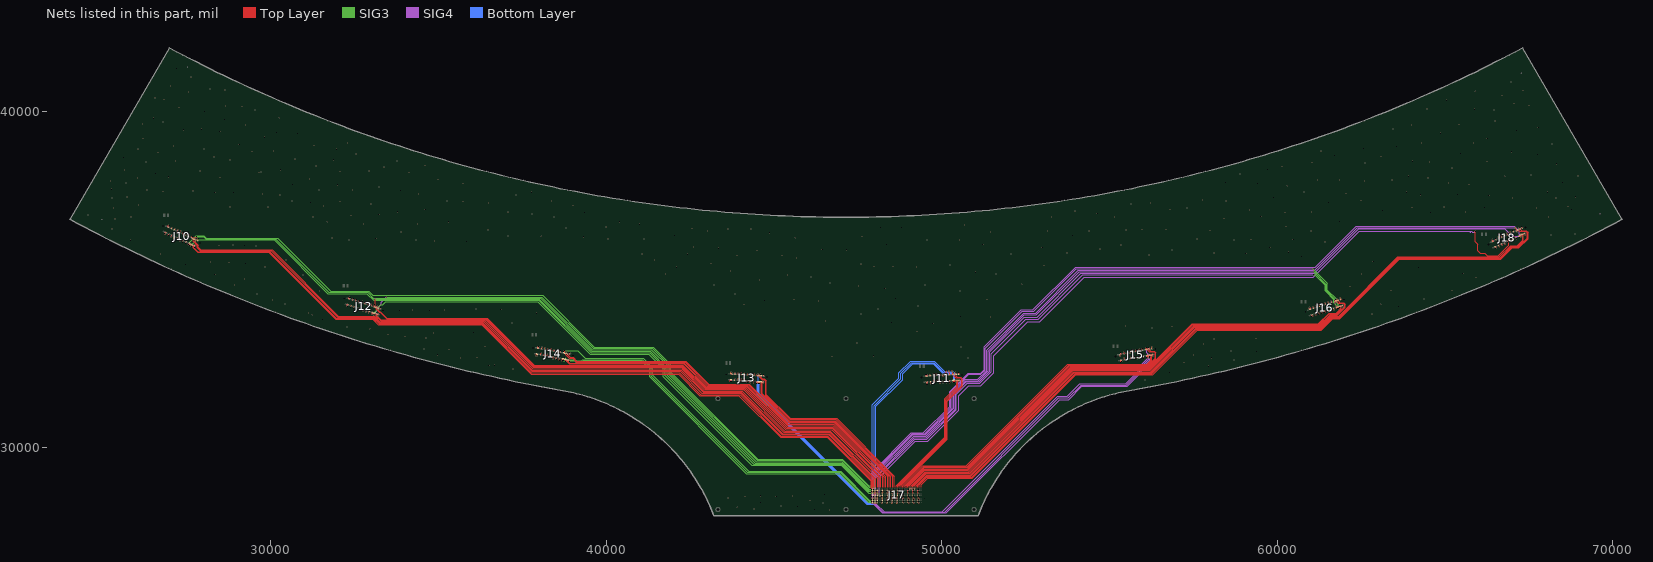
[diagram p0: the nets of this part, all layers, seen from the top]
# Altium PCB MISC86329.PcbDoc (part 10 of 11)
Units mil, origin at the board's own origin, x right, y up, seen from the top; angles counter-clockwise.
Board outline 46247.15 x 13937.21 mil, 6 copper layers (Top Layer, GND2, SIG3, SIG4, POWER5, Bottom Layer); 17 components, 210 nets, 908 pads, 1109 vias.

## Via types
v1: diameter 24, hole 12, Top Layer to Bottom Layer, 684 vias
v2: diameter 18, hole 9, Top Layer to Bottom Layer, 425 vias

## Nets (pads, with @x,y where several pads share a name; then routed paths per layer and width w, separated by ;. In a path a pad name is that pad's centre, name@x,y a point inside that pad or via, vN(x,y) a via of type N, cw(c..) or ccw(c..) an arc to the next point about the centre after c; other vN are vias at no path point) (continued)
DATAIN7P_CH7: J17.E25 J18.33 | length 23898
  Top Layer w5: v2(48164.09,28545) J17.E25@48187.89,28568.8 ; v2(65902.5,36445) 65896,36438.5 65896,36133.14 65970,36059.14 65970,35864 66043,35791 66184,35791 66255,35720 66589,35720 66898,36029 66898,36137.81 J18.33@66876.69,36159.11
  SIG4 w5: v2(48164.09,28545) 48144.09,28565 48144.09,29115.09 49215,30186 49587.14,30186 50507,31105.86 50507,31548 50807,31848 51168.14,31848 51552,32231.86 51552,32735 52571,33754 52922.14,33754 54244.14,35076 61077.14,35076 62441.14,36440 65673,36440 65741,36440 65746,36435 65746,36416.14 65751,36411.14 65761,36411.14 65766,36416.14 65766,36435 65771,36440 65776,36440 65786.86,36440 65815.86,36411 65882,36411 65896,36425 65896,36438.5
DGND: J10.5 J10.6 J10.7 J10.8 J10.13 J10.14 J10.19 J10.20 J10.25 J10.26 J10.31 J10.32 J10.37 J10.38 J10.43 J10.44 J10.49 J10.50 J10.55 J10.56 J10.61 J10.62 J10.67 J10.68 J11.5 J11.6 J11.7 J11.8 J11.13 J11.14 J11.19 J11.20 J11.25 J11.26 J11.31 J11.32 J11.37 J11.38 J11.43 J11.44 J11.49 J11.50 J11.55 J11.56 J11.61 J11.62 J11.67 J11.68 J12.5 J12.6 J12.7 J12.8 J12.13 J12.14 J12.19 J12.20 J12.25 J12.26 J12.31 J12.32 J12.37 J12.38 J12.43 J12.44 J12.49 J12.50 J12.55 J12.56 J12.61 J12.62 J12.67 J12.68 J13.5 J13.6 J13.7 J13.8 J13.13 J13.14 J13.19 J13.20 J13.25 J13.26 J13.31 J13.32 J13.37 J13.38 J13.43 J13.44 J13.49 J13.50 J13.55 J13.56 J13.61 J13.62 J13.67 J13.68 J14.5 J14.6 J14.7 J14.8 J14.13 J14.14 J14.19 J14.20 J14.25 J14.26 J14.31 J14.32 J14.37 J14.38 J14.43 J14.44 J14.49 J14.50 J14.55 J14.56 J14.61 J14.62 J14.67 J14.68 J15.5 J15.6 J15.7 J15.8 J15.13 J15.14 J15.19 J15.20 J15.25 J15.26 J15.31 J15.32 J15.37 J15.38 J15.43 J15.44 J15.49 J15.50 J15.55 J15.56 J15.61 J15.62 J15.67 J15.68 J16.5 J16.6 J16.7 J16.8 J16.13 J16.14 J16.19 J16.20 J16.25 J16.26 J16.31 J16.32 J16.37 J16.38 J16.43 J16.44 J16.49 J16.50 J16.55 J16.56 J16.61 J16.62 J16.67 J16.68 J17.A3 J17.A6 J17.A9 J17.A12 J17.A15 J17.A18 J17.A21 J17.A24 J17.A27 J17.B3 J17.B6 J17.B9 J17.B12 J17.B15 J17.B18 J17.B21 J17.B24 J17.B27 J17.C3 J17.C6 J17.C9 J17.C12 J17.C15 J17.C18 J17.C21 J17.C24 J17.C27 J17.D3 J17.D6 J17.D9 J17.D12 J17.D15 J17.D18 J17.D21 J17.D24 J17.D27 J17.E3 J17.E6 J17.E9 J17.E12 J17.E15 J17.E18 J17.E21 J17.E24 J17.E27 J17.F3 J17.F6 J17.F9 J17.F12 J17.F15 J17.F18 J17.F21 J17.F24 J17.F27 J17.G3 J17.G6 J17.G9 J17.G12 J17.G15 J17.G18 J17.G21 J17.G24 J17.G27 J17.H3 J17.H6 J17.H9 J17.H12 J17.H15 J17.H18 J17.H21 J17.H24 J17.H27 J17.J5 J17.J6 J17.J7 J17.J8 J18.5 J18.6 J18.7 J18.8 J18.13 J18.14 J18.19 J18.20 J18.25 J18.26 J18.31 J18.32 J18.37 J18.38 J18.43 J18.44 J18.49 J18.50 J18.55 J18.56 J18.61 J18.62 J18.67 J18.68 | length 12583.5
  Top Layer w5: J17.J8@49037.89,28768.8 v2(49061.69,28792.61) ; J17.F3@49287.89,28618.8 v2(49311.69,28642.61) ; J17.G3@49287.89,28668.8 v2(49311.69,28692.61) ; J17.H3@49287.89,28718.8 v2(49311.69,28742.61)
  Top Layer w20: v1(26840,36370) 26844,36376 J10.5@26861.63,36414.76 ; v1(26870,36360) 26873,36364 J10.7@26890.27,36401.67 ; J10.6@26935.3,36575.89 26952,36612 v1(26958,36627) ; v1(26956,36322) 26961,36330 J10.13@26976.21,36362.38 ; J10.8@26963.94,36562.79 26990,36616 v1(26990,36615) ; v1(27042,36280) 27049,36295 J10.19@27062.14,36323.09 ; J10.14@27049.87,36523.5 27066,36557 v1(27069,36563) ; v1(27126,36242) 27135,36257 J10.25@27148.07,36283.8 ; J10.20@27135.81,36484.21 27152,36519 v1(27156,36527) ; v1(27214,36201) 27219,36212 J10.31@27234,36244.51 ; J10.26@27221.74,36444.92 27238,36480 v1(27243,36490) ; v1(27298,36158) 27306,36175 J10.37@27319.94,36205.22 ; J10.32@27307.67,36405.64 27326,36445 v1(27331,36454) ; v1(27384,36119) 27390,36132 J10.43@27405.87,36165.94 ; J10.38@27393.6,36366.35 27414,36409 v1(27415,36411) ; v1(27471,36080) 27476,36091 J10.49@27491.8,36126.65 ; J10.44@27479.54,36327.06 27498,36368 v1(27502,36377) ; v1(27557,36042) 27563,36054 J10.55@27577.74,36087.36 ; J10.50@27565.47,36287.77 v1(27586,36332) ; J10.56@27651.4,36248.48 27671,36291 v1(27673,36295) ; v1(27654,35988) 27654,36027 J10.61@27663.67,36048.07 ; J10.62@27737.33,36209.19 27755,36247 v1(27756,36246) ; v1(27742,35960) 27742,35992 J10.67@27749.6,36008.78 ; J10.68@27823.27,36169.9 27846,36223 v1(27848,36226) ; v1(32268,34222) 32272,34232 J12.5@32282.85,34264.68 ; v1(32297,34208) 32302,34222 J12.7@32312.88,34255.17 ; J12.6@32336.33,34433.58 32351,34478 v1(32352,34479) ; J12.8@32366.36,34424.07 32380,34464 v1(32382,34471) ; v1(32388,34181) 32393,34194 J12.13@32402.96,34226.65 ; J12.14@32456.44,34395.55 32466,34426 v1(32471,34441) ; v1(32477,34150) 32481,34162 J12.19@32493.04,34198.13 ; J12.20@32546.52,34367.03 32559,34406 v1(32562,34414) ; v1(32567,34125) 32570,34131 J12.25@32583.12,34169.6 ; J12.26@32636.6,34338.5 32649,34375 v1(32653,34385) ; v1(32660,34098) 32664,34112 J12.31@32673.2,34141.08 ; J12.32@32726.68,34309.98 32740,34352 v1(32743,34361) ; v1(32750,34071) 32754,34083 J12.37@32763.28,34112.56 ; J12.38@32816.76,34281.46 32826,34311 v1(32834,34334) ; v1(32838,34034) 32842,34048 J12.43@32853.36,34084.03 ; J12.44@32906.84,34252.94 32919,34290 v1(32926,34310) ; v1(32927,34004) 32933,34022 J12.49@32943.44,34055.51 ; J12.50@32996.92,34224.41 33010,34264 v1(33016,34283) ; v1(33016,33978) 33020,33987 J12.55@33033.52,34026.99 ; J12.56@33087,34195.89 33097,34229 v1(33097,34256) ; v1(33111,33959) 33111,33961 J12.61@33123.6,33998.47 ; J12.62@33177.08,34167.37 33189,34204 v1(33193,34215) ; v1(33200,33927) 33203,33935 J12.67@33213.68,33969.94 ; J12.68@33267.16,34138.84 33279,34174 v1(33281,34176) ; v1(37915,32737) 37921,32763 J14.5@37925.69,32791.31 ; v1(37945,32733) 37949,32748 J14.7@37956.65,32785.53 ; J14.6@37958.19,32965.47 37965,33005 v1(37967,33014) ; J14.8@37989.15,32959.69 37994,32987 v1(37998,33008) ; J14.13@38049.54,32768.2 38049.54,32788.54 v1(38079,32818) ; J14.14@38082.04,32942.36 v1(38091,32993) ; J14.19@38142.42,32750.86 38142.42,32769.42 v1(38172,32799) ; J14.20@38174.92,32925.02 v1(38174.92,32978.92) ; J14.25@38235.31,32733.53 38235.31,32758.31 v1(38260,32783) ; J14.26@38267.81,32907.69 v1(38267.81,32957.19) ; J14.31@38328.19,32716.2 38328.19,32745.19 v1(38353,32770) ; J14.32@38360.69,32890.36 v1(38360.69,32938.31) ; v1(38421.08,32646.92) J14.37@38421.08,32698.87 ; J14.38@38453.58,32873.03 v1(38453.58,32921.58) ; v1(38513.96,32626.04) J14.43@38513.96,32681.53 ; J14.44@38546.46,32855.69 v1(38546.46,32904.54) ; v1(38606.85,32603.15) J14.49@38606.85,32664.2 ; J14.50@38639.35,32838.36 v1(38639.35,32889.35) ; v1(38685,32591) 38699.73,32605.73 J14.55@38699.73,32646.87 ; J14.56@38732.23,32821.03 v1(38732.23,32870.23) ; v1(38792.62,32562.38) J14.61@38792.62,32629.54 ; J14.62@38825.12,32803.7 v1(38825.12,32851.88) ; J14.67@38885.5,32612.2 38885.5,32582.5 v1(38911,32557) ; J14.68@38918,32786.36 v1(38918,32833) ; v1(43703,31968) J13.5@43706.03,32016.6 ; J13.6@43717.06,32193.43 43720,32239 v1(43721,32250) ; v1(43735,31963) 43735,31971 J13.7@43737.46,32014.64 ; J13.8@43748.5,32191.46 43751,32234 v1(43751,32239) ; J13.13@43831.77,32008.76 v1(43834,32052) ; J13.14@43842.8,32185.58 43846,32231 v1(43846,32232) ; J13.19@43926.07,32002.88 43929,32049 v1(43929,32050) ; J13.20@43937.11,32179.7 43940,32223 v1(43940,32227) ; J13.25@44020.38,31996.99 44023,32042 v1(44024,32047) ; J13.26@44031.41,32173.81 44034,32217 v1(44035,32224) ; J13.31@44114.68,31991.11 v1(44118,32044) ; J13.32@44125.72,32167.93 44130,32214 v1(44130,32217) ; v1(44206,31936) 44207,31947 J13.37@44208.99,31985.22 ; J13.38@44220.02,32162.05 44223,32207 v1(44224,32209) ; v1(44300,31928) 44300,31933 J13.43@44303.29,31979.34 ; J13.44@44314.33,32156.16 44317,32198 v1(44318,32203) ; v1(44394,31922) 44395,31935 J13.49@44397.6,31973.46 ; J13.50@44408.63,32150.28 44412,32196 v1(44413,32200) ; v1(44488,31915) J13.55@44491.9,31967.57 ; J13.56@44502.94,32144.4 v1(44505,32184) ; v1(44583,31914) 44584,31924 J13.61@44586.21,31961.69 ; J13.62@44597.24,32138.51 v1(44600,32186) ; v1(44678,31908) 44679,31918 J13.67@44680.51,31955.81 ; J13.68@44691.54,32132.63 44694,32173 v1(44695,32181) ; v2(48064.09,28345) J17.A27@48087.89,28368.8 ; v2(48064.09,28395) J17.B27@48087.89,28418.8 ; v2(48064.09,28445) J17.C27@48087.89,28468.8 ; v2(48064.09,28495) J17.D27@48087.89,28518.8 ; v2(48064.09,28545) J17.E27@48087.89,28568.8 ; v2(48064.09,28642.61) J17.F27@48087.89,28618.8 ; v2(48064.09,28692.61) J17.G27@48087.89,28668.8 ; v2(48064.09,28742.61) J17.H27@48087.89,28718.8 ; v2(48214.09,28345) J17.A24@48237.89,28368.8 ; v2(48214.09,28395) J17.B24@48237.89,28418.8 ; v2(48214.09,28445) J17.C24@48237.89,28468.8 ; v2(48214.09,28495) J17.D24@48237.89,28518.8 ; v2(48214.09,28545) J17.E24@48237.89,28568.8 ; v2(48214.09,28642.61) J17.F24@48237.89,28618.8 ; v2(48214.09,28692.61) J17.G24@48237.89,28668.8 ; v2(48214.09,28742.61) J17.H24@48237.89,28718.8 ; v2(48364.09,28345) J17.A21@48387.89,28368.8 ; v2(48364.09,28395) J17.B21@48387.89,28418.8 ; v2(48364.09,28445) J17.C21@48387.89,28468.8 ; v2(48364.09,28495) J17.D21@48387.89,28518.8 ; v2(48364.09,28545) J17.E21@48387.89,28568.8 ; v2(48364.09,28642.61) J17.F21@48387.89,28618.8 ; v2(48364.09,28692.61) J17.G21@48387.89,28668.8 ; v2(48364.09,28742.61) J17.H21@48387.89,28718.8 ; v2(48514.09,28345) J17.A18@48537.89,28368.8 ; v2(48514.09,28395) J17.B18@48537.89,28418.8 ; v2(48514.09,28445) J17.C18@48537.89,28468.8 ; v2(48514.09,28495) J17.D18@48537.89,28518.8 ; v2(48514.09,28545) J17.E18@48537.89,28568.8 ; v2(48514.09,28642.61) J17.F18@48537.89,28618.8 ; v2(48514.09,28692.61) J17.G18@48537.89,28668.8 ; v2(48514.09,28742.61) J17.H18@48537.89,28718.8 ; v2(48664.09,28345) J17.A15@48687.89,28368.8 ; v2(48664.09,28395) J17.B15@48687.89,28418.8 ; v2(48664.09,28445) J17.C15@48687.89,28468.8 ; v2(48664.09,28495) J17.D15@48687.89,28518.8 ; v2(48664.09,28545) J17.E15@48687.89,28568.8 ; J17.F15@48687.89,28618.8 v2(48711.69,28642.61) ; J17.G15@48687.89,28668.8 v2(48711.69,28692.61) ; J17.H15@48687.89,28718.8 v2(48711.69,28742.61) ; J17.A12@48837.89,28368.8 v2(48861.69,28345) ; J17.B12@48837.89,28418.8 v2(48861.69,28395) ; J17.C12@48837.89,28468.8 v2(48861.69,28445) ; J17.D12@48837.89,28518.8 v2(48861.69,28495) ; J17.E12@48837.89,28568.8 v2(48861.69,28545) ; J17.F12@48837.89,28618.8 v2(48861.69,28642.61) ; J17.G12@48837.89,28668.8 v2(48861.69,28692.61) ; J17.H12@48837.89,28718.8 v2(48861.69,28742.61) ; J17.A9@48987.89,28368.8 v2(49011.69,28345) ; J17.B9@48987.89,28418.8 v2(49011.69,28395) ; J17.C9@48987.89,28468.8 v2(49011.69,28445) ; J17.D9@48987.89,28518.8 v2(49011.69,28495) ; J17.E9@48987.89,28568.8 v2(49011.69,28545) ; J17.F9@48987.89,28618.8 v2(49011.69,28642.61) ; J17.G9@48987.89,28668.8 v2(49011.69,28692.61) ; J17.H9@48987.89,28718.8 v2(49011.69,28742.61) ; J17.J8@49037.89,28768.8 v2(49061.69,28792.61) ; J17.J7@49087.89,28768.8 v2(49111.69,28792.61) ; J17.A6@49137.89,28368.8 v2(49161.69,28345) ; J17.B6@49137.89,28418.8 v2(49161.69,28395) ; J17.C6@49137.89,28468.8 v2(49161.69,28445) ; J17.D6@49137.89,28518.8 v2(49161.69,28495) ; J17.E6@49137.89,28568.8 v2(49161.69,28545) ; J17.F6@49137.89,28618.8 v2(49161.69,28642.61) ; J17.G6@49137.89,28668.8 v2(49161.69,28692.61) ; J17.H6@49137.89,28718.8 v2(49161.69,28742.61) ; J17.J6@49137.89,28768.8 v2(49161.69,28792.61) ; J17.J5@49187.89,28768.8 v2(49211.69,28792.61) ; J17.A3@49287.89,28368.8 v2(49311.69,28345) ; J17.B3@49287.89,28418.8 v2(49311.69,28395) ; J17.C3@49287.89,28468.8 v2(49311.69,28445) ; J17.D3@49287.89,28518.8 v2(49311.69,28495) ; J17.E3@49287.89,28568.8 v2(49311.69,28545) ; J17.F3@49287.89,28618.8 v2(49311.69,28642.61) ; J17.G3@49287.89,28668.8 v2(49311.69,28692.61) ; J17.H3@49287.89,28718.8 v2(49311.69,28742.61) ; v1(49526,32172) 49525,32168 J11.6@49527.1,32128.97 ; J11.5@49537.7,31952.12 49541,31892 v1(49542,31888) ; v1(49555,32178) 49556,32171 J11.8@49558.54,32130.85 ; J11.7@49569.14,31954.01 49573,31892 v1(49574,31886) ; v1(49651,32183) 49651,32177 J11.14@49652.86,32136.51 ; J11.13@49663.45,31959.66 49667,31901 v1(49667,31896) ; v1(49744,32187) J11.20@49747.17,32142.16 ; v1(49754,32026) J11.19@49757.77,31965.31 ; v1(49839,32198) 49839,32197 J11.26@49841.49,32147.81 ; v1(49849,32028) 49849,32025 J11.25@49852.09,31970.97 ; v1(49933,32202) J11.32@49935.81,32153.47 ; J11.31@49946.41,31976.62 49949,31924 v1(49949,31923) ; J11.38@50030.13,32159.12 50032,32118 v1(50034,32112) ; J11.37@50040.73,31982.27 50044,31930 v1(50045,31926) ; v1(50118,32290) 50118,32288 J11.44@50124.45,32164.77 ; J11.43@50135.05,31987.92 50138,31938 v1(50139,31930) ; v1(50213,32285) 50213,32279 J11.50@50218.77,32170.43 ; J11.49@50229.37,31993.58 50232,31946 v1(50233,31936) ; v1(50307,32287) 50307,32282 J11.56@50313.09,32176.08 ; J11.55@50323.69,31999.23 50327,31961 v1(50328,31956) ; v1(50404,32244) 50404,32240 J11.62@50407.41,32181.73 ; J11.61@50418.01,32004.88 50420,31963 v1(50421,31956) ; v1(50499,32234) J11.68@50501.73,32187.38 ; J11.67@50512.33,32010.54 50515,31970 v1(50515,31968) ; J15.6@55301.68,32773.06 55309,32733 v1(55310,32727) ; v1(55323,32828) 55325,32821 J15.8@55332.65,32778.76 ; v1(55333.75,32539.75) J15.5@55333.75,32598.82 ; v1(55364.73,32561.73) J15.7@55364.73,32604.52 ; v1(55418,32842) 55421,32823 J15.14@55425.58,32795.87 ; v1(55426,32670) 55457.65,32638.35 J15.13@55457.65,32621.63 ; J15.20@55518.51,32812.97 55518.51,32766.49 55518.99,32766.01 v1(55519,32765) ; v1(55526,32683) 55550.58,32658.42 J15.19@55550.58,32638.73 ; J15.26@55611.44,32830.08 v1(55611.44,32876.44) ; v1(55621,32702) 55643.51,32679.49 J15.25@55643.51,32655.84 ; J15.32@55704.36,32847.18 v1(55704.36,32900.36) ; J15.31@55736.44,32672.95 v1(55736.44,32719.44) ; J15.38@55797.29,32864.29 v1(55797.29,32917.29) ; v1(55829.36,32643.36) J15.37@55829.36,32690.05 ; J15.44@55890.22,32881.39 v1(55890.22,32932.22) ; v1(55922.29,32648.29) J15.43@55922.29,32707.16 ; J15.50@55983.14,32898.5 v1(55983.14,32945.14) ; v1(56015.22,32662.22) J15.49@56015.22,32724.26 ; J15.56@56076.07,32915.61 v1(56076.07,32962.07) ; v1(56108.14,32689.14) J15.55@56108.14,32741.37 ; J15.62@56169,32932.71 v1(56169,32978) ; v1(56201.07,32711.07) J15.61@56201.07,32758.47 ; J15.68@56261.92,32949.82 v1(56261.92,32997.92) ; v1(56294,32726) J15.67@56294,32775.58 ; v1(60943,34154) 60945,34147 J16.6@60954.72,34116.09 ; v1(60964,34185) 60965.24,34182.1 60970,34171 ; v1@60965,34182 60976.06,34152.34 J16.8@60984.77,34125.53 ; J16.5@61007.79,33947.06 61020,33910 v1(61023,33902) ; J16.7@61037.84,33956.5 61050,33920 v1(61052,33915) ; v1(61060,34199) 61064,34187 J16.14@61074.92,34153.83 ; J16.13@61127.99,33984.8 61139,33951 v1(61141,33947) ; v1(61150,34230) 61154,34218 J16.20@61165.07,34182.13 ; J16.19@61218.14,34013.1 61228,33981 v1(61231,33972) ; v1(61238,34261) 61242,34253 J16.26@61255.22,34210.44 ; J16.25@61308.29,34041.4 61320,34005 v1(61321,34000) ; v1(61331,34281) 61331,34282 J16.32@61345.37,34238.74 ; J16.31@61398.44,34069.71 61409,34038 v1(61415,34021) ; v1(61418,34320) 61421,34312 J16.38@61435.52,34267.04 ; J16.37@61488.59,34098.01 61499,34067 v1(61507,34046) ; v1(61508,34345) 61515,34329 J16.44@61525.67,34295.34 ; J16.43@61578.74,34126.31 61591,34089 v1(61596,34075) ; v1(61602,34366) 61606,34355 J16.50@61615.82,34323.65 ; J16.49@61668.89,34154.62 61678,34124 61682,34110 v1(61684,34104) ; J16.56@61705.97,34351.95 61717,34320 v1(61721,34309) ; v1(61745,34224) 61748,34216 J16.55@61759.04,34182.92 ; v1(61782,34423) J16.62@61796.12,34380.25 ; J16.61@61849.19,34211.22 61860,34181 v1(61861,34177) ; v1(61871,34457) J16.68@61886.27,34408.56 ; J16.67@61939.34,34239.53 61952,34200 v1(61954,34195) ; v1(66383,36181) 66387,36171 J18.6@66401.96,36138.05 ; v1(66405,36207) 66410,36197 J18.8@66430.63,36151.07 ; J18.5@66475.23,35976.74 66491,35943 v1(66497,35930) ; v1(66498,36229) 66500,36224 J18.14@66516.66,36190.15 ; J18.7@66503.91,35989.77 66522,35951 v1(66524,35947) ; v1(66583,36273) 66585,36266 J18.20@66602.69,36229.23 ; J18.13@66589.93,36028.85 66604,35999 v1(66610,35987) ; v1(66670,36307) 66674,36299 J18.26@66688.72,36268.31 ; J18.19@66675.96,36067.93 v1(66697,36024) ; v1(66756,36347) 66758,36343 J18.32@66774.75,36307.39 ; J18.25@66761.99,36107.01 66780,36068 v1(66781,36064) ; v1(66840,36390) 66843,36385 J18.38@66860.78,36346.47 ; J18.31@66848.02,36146.08 66866,36109 v1(66868,36105) ; v1(66927,36429) 66930,36422 J18.44@66946.8,36385.54 ; J18.37@66934.05,36185.16 66954,36143 v1(66955,36142) ; v1(67014,36467) 67016,36462 J18.50@67032.83,36424.62 ; J18.43@67020.08,36224.24 v1(67039,36185) ; J18.49@67106.1,36263.32 67122,36230 v1(67127,36222) ; J18.56@67118.86,36463.7 67134,36433 v1(67137,36427) ; v1(67184,36546) 67187,36540 J18.62@67204.89,36502.78 ; J18.55@67192.13,36302.4 67209,36267 v1(67214,36258) ; v1(67260,36381) 67263,36374 J18.61@67278.16,36341.48 ; v1(67271,36584) 67276,36574 J18.68@67290.92,36541.86 ; J18.67@67364.19,36380.56 67383,36343 v1(67387,36333)
  other v1: 46658,28143 46206,28159 44415,28164 43908,28221 45709,28247 45207,28258 46459,28346 44607,28366 46076,28428 43639,28496 44136,28547 45072,28547 45559,28553 44601,28563 46506,28604 56058,32008 56783,32233 37223,32334 57950,32423 36505,32446 36677,32452 57216,32530 58715,32605 35667,32666 50786,32672 58039,32675 36154,32684 46731,32718 47974,32737 57499,32759 34972,32767 59378,32861 58622,32874 35322,32922 34579,32940 50579,32999 36398,33017 57804,33087 47470,33111 58123,33233 59360,33250 34627,33260 34003,33314 33504,33367 34853,33415 36047,33427 49262,33464 32957,33540 56270,33560 32286,33593 56863,33613 55479,33626 49733,33699 37200,33706 48507,33728 46544,33775 31549,33813 51453,33887 50555,33906 31246,33957 62826,33972 47591,33980 37930,34003 31129,34011 33849,34086 34734,34086 34229,34104 35191,34104 36861,34110 36124,34128 48099,34132 63611,34205 49296,34221 44104,34261 63082,34269 30433,34282 46329,34373 44721,34382 30061,34399 45604,34411 51354,34411 64372,34429 48620,34438 29599,34579 43843,34579 50544,34661 31464,34664 63387,34677 65205,34685 48304,34745 62169,34805 47526,34812 43211,34840 49508,34840 28923,34845 52387,34867 46674,34902 44572,34999 29221,35026 65918,35062 46105,35083 45400,35140 30965,35143 28339,35159 41767,35166 51619,35166 62505,35166 65525,35182 51003,35224 43709,35256 64204,35366 42094,35373 49246,35383 29832,35387 47984,35401 48554,35401 53052,35420 50252,35435 27474,35450 47595,35461 43122,35486 29258,35488 28764,35515 28211,35526 62858,35542 41440,35586 30465,35595 45672,35652 60717,35697 43899,35719 45245,35728 56184,35739 42421,35760 52068,35763 26725,35771 41079,35773 59061,35782 58121,35796 53736,35806 60339,35819 44493,35870 56868,35883 47164,35894 46441,35897 54720,35909 43348,35938 59776,35957 52998,35961 42601,35980 29572,36004 28461,36025 29232,36025 28886,36036 55335,36037 51225,36055 48358,36056 61418,36132 35837,36137 34885,36155 25831,36176 49557,36180 58710,36182 50527,36187 32344,36190 34338,36190 60476,36196 59216,36203 41126,36214 57615,36217 40058,36221 33138,36226 31841,36243 45637,36252 39324,36281 47622,36286 38069,36296 37081,36305 42034,36321 53901,36324 68159,36339 68872,36367 44871,36402 51453,36423 33896,36428 43020,36448 61011,36448 53151,36456 54398,36456 57992,36467 55500,36479 36481,36490 56680,36500 55968,36503 44310,36514 43627,36517 25274,36520 42564,36524 38810,36541 48177,36563 48805,36563 40005,36574 60257,36592 50674,36632 40993,36654 32777,36656 34382,36667 31691,36728 35308,36728 40399,36728 61853,36736 25365,36818 58415,36827 68077,36866 38450,36868 53274,36873 55147,36875 25849,36877 31267,36878 59506,36891 32405,36914 24563,36932 33226,36940 37796,36958 54634,36976 64561,37007 39357,37008 60225,37009 37081,37011 61025,37016 65611,37016 33782,37028 53967,37041 63130,37066 59166,37073 68763,37093 56801,37096 34611,37099 57307,37136 25319,37139 67718,37142 66176,37150 64014,37157 29926,37162 64975,37167 28792,37176 68660,37183 31575,37196 39017,37208 26065,37225 32988,37258 55641,37261 56217,37283 36499,37284 31197,37302 61522,37306 32070,37337 35731,37337 38376,37342 30643,37343 35265,37347 58478,37349 62499,37367 57770,37374 67012,37434 25281,37437 68297,37438 59884,37457 25732,37467 68880,37475 66300,37510 30278,37521 37311,37522 64263,37533 65373,37545 29758,37551 34408,37558 62046,37569 28903,37597 28340,37601 63855,37607 68048,37608 37782,37609 60801,37620 26802,37635 27688,37651 33879,37664 31444,37672 32449,37672 26313,37674 25266,37696 33235,37761 60296,37802 32001,37830 30657,37837 65707,37841 35740,37867 59414,37874 25694,37880 65104,37889 58460,37895 68497,37897 62604,37938 25235,37941 61197,37972 61853,37978 63425,37978 34990,37990 31161,38008 26038,38033 64490,38039 28498,38048 26962,38071 63908,38084 66778,38084 68959,38099 67564,38116 58892,38153 26580,38162 34126,38193 29656,38199 29720,38208 32070,38228 27909,38239 32944,38246 25656,38269 30301,38277 59712,38290 65205,38322 33385,38352 60141,38371 31364,38387 34603,38407 68316,38458 62609,38474 61036,38490 64539,38506 26290,38514 66249,38522 64028,38532 33773,38537 27176,38544 28796,38575 31878,38577 30736,38590 25625,38644 28319,38665 63095,38672 61699,38700 67751,38733 32555,38749 65454,38766 26649,38789 66979,38814 29453,38820 61300,38830 30086,38839 26053,38888 31964,38890 28016,38896 62566,38913 63551,38974 27115,38980 31294,38996 29071,39033 68189,39050 65841,39072 64301,39074 32299,39075 66257,39204 26206,39209 29819,39247 30805,39354 64863,39367 30184,39389 28490,39415 67126,39447 27405,39469 27948,39484 63449,39496 67775,39537 29262,39606 64000,39612 65415,39625 26183,39637 26802,39706 66494,39734 28632,39772 26519,39813 30263,39828 28039,40011 29537,40057 66453,40063 65876,40081 64463,40097 27275,40134 29155,40157 28658,40172 67499,40194 67050,40255 65040,40348 26832,40370 26557,40424 66695,40494 27558,40600 65900,40616 67324,40643 28639,40655 28200,40684 27016,40775 66963,40892 27627,41035 27199,41295
  other v2: 49311.69,28642.61 49311.69,28692.61 49311.69,28742.61 49061.69,28792.61
IO0_CH0: J10.57 J17.G28 | length 24027.9
  Top Layer w5: v2(27593,36021) 27593,36050 27606.38,36063.38 J10.57@27606.38,36074.26 ; v2(48014.09,28692.61) J17.G28@48037.89,28668.8
  SIG3 w5: v2@27593,36023 27593,36110.58 27788.42,36306 28018,36306 28091,36233 28163,36233 ; 28159,36233 28163,36233 ; v2(48014.09,28692.61) 47997.59,28709.11 47997.59,28793.41 47972,28819 47954,28819 47940,28833 47940,28851 47924,28867 47829,28867 47040,29656 44524,29656 41934,32246 41934,32465 41404,32995 39651,32995 38111,34535 33044,34535 32928,34651 31798,34651 30216,36233 28163,36233
IO0_CH1: J12.57 J17.F28 | length 17930.8
  Top Layer w5: v2(33055,33969) 33055,34008.93 J12.57@33063.55,34017.48 ; v2(48014.09,28642.61) J17.F28@48037.89,28618.8
  SIG4 w5: v2@33059,33972 33225,34138 33225,34187 33303,34265 33303,34332 v2(33457,34486)
  SIG3 w5: v2(33457,34486) 38088,34486 39615,32959 41379,32959 41894,32444 41894,32221 44498,29617 47032,29617 47836,28813 47925,28813 47939,28799 47939,28785 47955,28769 47973,28769 47986,28756 47986,28670.69 v2(48014.09,28642.61)
IO0_CH2: J14.57 J17.B28 | length 11301.6
  Top Layer w5: v2@38725,32593 38725,32634 38730.69,32639.69 J14.57@38730.69,32641.09 ; v2(48014.09,28395) J17.B28@48037.89,28418.8
  SIG4 w5: v2@38723,32591 v2(38724,32590)
  SIG3 w5: v2(38724,32590) 39053,32590 39080,32563 39290,32563 39317,32590 41054,32590 41298,32346 41298,32105 44176,29227 46957,29227 47819,28365 47984.09,28365 v2(48014.09,28395)
IO0_CH3: J13.57 J17.A28 | length 5297.8
  Top Layer w5: v2@44523.34,31910.34 J13.57@44523.34,31965.61 ; v2(48014.09,28345) J17.A28@48037.89,28368.8
  Bottom Layer w5: v2@44520,31906 44510,31896 44510,31572 47772,28310 47979.09,28310 v2(48014.09,28345) ; v2@44521,31906 v2(44521,31907)
IO0_CH4: J11.57 J17.H28 | length 5891.1
  Top Layer w5: v2(48014.09,28742.61) J17.H28@48037.89,28718.8 ; v2(50355.13,31939.13) J11.57@50355.13,32001.12
  Bottom Layer w5: v2(48014.09,28742.61) 48038,28766.52 48038,31230 48836,32028 48836,32193 49139,32496 49746,32496 50046,32196 50319,32196 50355.13,32159.87 v2(50355.13,31939.13)
IO0_CH5: J15.57 J17.C28 | length 10400.7
  Top Layer w5: v2(48014.09,28445) J17.C28@48037.89,28468.8 ; v2(56139.12,32666.12) J15.57@56139.12,32747.07
  SIG4 w5: v2(48014.09,28445) 48042,28417.09 48042,28331 48286,28087 50021,28087 53461,31527 53747,31527 54116,31896 55482,31896 55857,32271 55857,32385 v2@56138,32666
IO0_CH6: J16.57 J17.D28 | length 18151.7
  Top Layer w5: v2(48014.09,28495) J17.D28@48037.89,28518.8 ; v2(61789.09,34137.91) J16.57@61789.09,34192.35
  SIG4 w5: v2(48014.09,28495) 48042,28522.91 48042,29094 49199,30251 49560,30251 50441,31132 50441,31591 50769,31919 51141,31919 51482,32260 51482,32795 52509,33822 52884,33822 54210,35148 v2(61074,35148)
  SIG3 w5: v2@61070,35148 v2(61074,35148) 61109,35148 61422,34835 61422,34671 61686.5,34406.5 61686.5,34315.92 61712.92,34289.5 61713.5,34289.5 61789,34214 ; v2(61789.09,34137.91) 61789.09,34214
IO0_CH7: J17.E28 J18.57 | length 23718.6
  Top Layer w5: v2(48014.09,28545) J17.E28@48037.89,28568.8 ; J18.57@67220.81,36315.42 67220.81,36302.19 v2@67257,36266 ; v2(67258,36266) v2@67257,36266 ; v2@67259,36264 v2@67257,36266
  SIG4 w5: v2(48014.09,28545) 48032,28562.91 48032,28888 ; 48032,28895 48032,28888 ; v2(67258,36266) 67223,36301 67003,36301 66784,36520 62430,36520 61101,35191 54143,35191 52842,33890 52464,33890 51425,32851 51425,32268 51116,31959 50739,31959 50398,31618 50398,31149 49540,30291 49178,30291 48032,29145 48032,28888
IO1_CH0: J10.58 J17.G29 | length 23611.7
  Top Layer w5: J10.58@27690,36245.34 27715.66,36271 27786,36271 v2(27799,36284) ; v2(47964.09,28692.61) J17.G29@47987.89,28668.8
  SIG3 w5: v2@27800,36283 28012,36283 28084,36211 30156,36211 31744,34623 32896,34623 33066,34453 38055,34453 39586,32922 41344,32922 41846,32420 41846,32204 44477,29573 47028,29573 47837,28764 47924,28764 47946,28742 47946,28710.69 v2(47964.09,28692.61)
IO1_CH1: J12.58 J17.F29 | length 17648.8
  Top Layer w5: J12.58@33117.03,34186.38 33117.03,34419.03 v2@33121,34423 ; v2(47964.09,28642.61) J17.F29@47987.89,28618.8
  SIG3 w5: v2@33117,34423 38016,34423 39574,32865 41316,32865 41796,32385 41796,32179 44443,29532 47022,29532 47840,28714 47918,28714 47941.85,28690.15 47941.85,28664.85 v2(47964.09,28642.61)
  other v2: 33116,34424
IO1_CH2: J14.58 J17.B29 | length 11294.3
  Top Layer w5: J14.58@38763.19,32815.25 38768,32820.06 38768,32884 v2@38766,32886 ; v2(47964.09,28395) J17.B29@47987.89,28418.8
  SIG3 w5: v2(38768,32889) 39152,32889 39386,32655 41102,32655 41387,32370 41387,32149 44244,29292 46987,29292 47860,28419 47940.09,28419 v2(47964.09,28395)
IO1_CH3: J13.58 J17.A29 | length 5474
  Top Layer w5: J13.58@44534.37,32142.43 v2(44534.37,32193.37) ; v2(47964.09,28345) J17.A29@47987.89,28368.8
  Bottom Layer w5: v2@44535,32189 44538.27,32185.73 44538.27,31585.73 47799,28325 47944.09,28325 v2(47964.09,28345)
IO1_CH4: J11.58 J17.H29 | length 5714.2
  Top Layer w5: v2(47964.09,28742.61) J17.H29@47987.89,28718.8 ; J11.58@50344.53,32177.96 v2(50344.53,32230.47)
  Bottom Layer w5: v2(47964.09,28742.61) 47988,28766.52 47988,31252 48781,32045 48781,32208 49107,32534 49765,32534 50068.53,32230.47 v2(50344.53,32230.47)
IO1_CH5: J15.58 J17.C29 | length 10818.9
  Top Layer w5: v2(47964.09,28445) J17.C29@47987.89,28468.8 ; J15.58@56107.05,32921.31 v2(56107.05,32976.05)
  SIG4 w5: v2(47964.09,28445) 47990,28419.09 47990,28330 48249,28071 50085,28071 53495,31481 53773,31481 54153,31861 55504,31861 55900,32257 55900,32370 56166,32636 56166,32772 56108,32830 56108,32975 v2@56109,32976
IO1_CH6: J16.58 J17.D29 | length 18077.8
  Top Layer w5: v2(47964.09,28495) J17.D29@47987.89,28518.8 ; v2(61730,34411) 61730,34367.41 J16.58@61736.02,34361.38
  SIG4 w5: v2(47964.09,28495) 47993,28523.91 47993,29169 49163,30339 49525,30339 50354,31168 50354,31629 50723,31998 51091,31998 51382,32289 51382,32873 52462,33953 52817,33953 54099,35235 v2(61081,35235)
  SIG3 w5: v2@61080,35235 61461,34854 61461,34680 v2(61730,34411)
IO1_CH7: J17.E29 J18.58 | length 23589.8
  Top Layer w5: v2(47964.09,28545) J17.E29@47987.89,28568.8 ; v2@67078.13,36546.13 67091.13,36533.13 J18.58@67147.54,36476.73
  SIG4 w5: v2(47964.09,28545) 47981,28561.91 47981,28888 ; 47981,28892 47981,28888 ; v2(67078,36545) 67066,36557 62389,36557 61111,35279 54069,35279 52799,34009 52446,34009 51338,32901 51338,32294 51081,32037 50704,32037 50309,31642 50309,31174 49514,30379 49138,30379 47981,29222 47981,28888
IO2_CH0: J10.59 J17.G30 | length 23701.8
  Top Layer w5: v2(27626,36006) 27626,36052.14 J10.59@27635.02,36061.17 ; v2(47914.09,28692.61) J17.G30@47937.89,28668.8
  SIG3 w5: v2@27629,36008 27809,36188 27959,36188 ; 27952,36188 27959,36188 ; 28223,36188 28228,36188 ; v2@47920,28690 47917.39,28692.61 v2(47914.09,28692.61) 47816.39,28692.61 47005,29504 44394,29504 41750,32148 41750,32363 41294,32819 39556,32819 37989,34386 33077,34386 32874,34589 31708,34589 30109,36188 28228,36188 ; 27959,36188 28228,36188
IO2_CH1: J12.59 J17.F30 | length 17670.1
  Top Layer w5: v2(33086,33942) 33086,34000.4 J12.59@33093.57,34007.97 ; v2(47914.09,28642.61) J17.F30@47937.89,28618.8
  SIG3 w5: v2@33084,33946 33084,33998 33217,34131 33217,34180 33293,34256 33342,34256 33435,34349 33532,34349 ; 33528,34349 33532,34349 ; v2(47914.09,28642.61) 47828.39,28642.61 47001,29470 44341,29470 41705,32106 41705,32351 41276,32780 39530,32780 37961,34349 33532,34349
IO2_CH2: J14.59 J17.B30 | length 11163.8
  Top Layer w5: J14.59@38761.66,32635.31 38766,32639.66 v2(38766,32677) ; v2(47914.09,28395) J17.B30@47937.89,28418.8
  SIG3 w5: v2@38769,32674 38822,32621 39056,32621 39096,32581 39266,32581 39309,32624 41075,32624 41342,32357 41342,32129 44213,29258 46975,29258 47838,28395 v2(47914.09,28395)
IO2_CH3: J13.59 J17.A30 | length 5095.5
  Top Layer w5: v2(44554.77,31905.23) J13.59@44554.77,31963.65 ; v2(47914.09,28345) J17.A30@47937.89,28368.8
  Bottom Layer w5: v2@44554,31905 44565,31894 44565,31606 47826,28345 v2(47914.09,28345)
IO2_CH4: J11.59 J17.H30 | length 6147.6
  Top Layer w5: v2(47914.09,28742.61) J17.H30@47937.89,28718.8 ; v2(50386.57,31939.57) J11.59@50386.57,32003
  Bottom Layer w5: v2(47914.09,28742.61) 47937,28765.52 47937,31280 48726,32069 48726,32226 49076,32576 49773,32576 50089,32260 50342,32260 50386.57,32215.43 v2(50386.57,31939.57)
IO2_CH5: J15.59 J17.C30 | length 10634.5
  Top Layer w5: v2(47914.09,28445) J17.C30@47937.89,28468.8 ; J15.59@56170.09,32752.77 56170.09,32734.91 56178,32727 56178,32693 v2(56196,32675)
  SIG4 w5: v2(47914.09,28445) 47939,28420.09 47939,28340 48226,28053 50134,28053 53513,31432 53782,31432 54171,31821 55525,31821 55946,32242 55946,32358 56197,32609 v2@56197,32674
IO2_CH6: J16.59 J17.D30 | length 18649.1
  Top Layer w5: v2(47914.09,28495) J17.D30@47937.89,28518.8 ; v2(61819.14,34137.14) J16.59@61819.14,34201.79
  SIG4 w5: v2(47914.09,28495) 47944,28524.91 47944,29237 49120,30413 49498,30413 50271,31186 50271,31657 50801,32187 51168,32187 51291,32310 51291,32957 52397,34063 52746,34063 54010,35327 v2(61062,35327)
  SIG3 w5: v2@61061,35324 61495,34890 61495,34692 61757,34430 61757,34325 61819.14,34262.86 v2(61819.14,34137.14)
IO2_CH7: J17.E30 J18.59 | length 24056.1
  Top Layer w5: v2(47914.09,28545) J17.E30@47937.89,28568.8 ; J18.59@67249.48,36328.45 67249.48,36312.52 v2@67283,36279
  SIG4 w5: v2(47914.09,28545) 47932,28562.91 47932,29271 49100,30439 49458,30439 50237,31218 50237,31662 50791,32216 51161,32216 51267,32322 51267,33005 52365,34103 52713,34103 53988,35378 61137,35378 62349,36590 67066,36590 67214,36442 67214,36349 v2(67283,36280)
IO3_CH0: J10.60 J17.J29 | length 23613.6
  Top Layer w5: J10.60@27708.69,36222.29 27702,36215.6 27702,36141 27822,36021 27822,35955 27911,35866 28065,35866 ; 28069,35866 28065,35866 ; J17.J29@47989,28768 47965,28792 47965,29041 46630,30376 45254,30376 44014,31616 42857,31616 42205,32268 37785,32268 36330,33723 33246,33723 33081,33888 31998,33888 30020,35866 28065,35866
IO3_CH1: J12.60 J17.K26 | length 17419.5
  Top Layer w5: J12.60@33147.05,34176.87 33147.05,34115.95 33236,34027 33272,34027 33466,33833 36434,33833 37838,32429 42275,32429 42949,31755 44134,31755 45353,30536 46717,30536 48137.89,29115.11 J17.K26@48137.89,28818.8
IO3_CH2: J14.60 J17.K22 | length 11405.8
  Top Layer w5: J14.60@38794.15,32809.47 38794.15,32770.85 38906,32659 39003,32659 39116,32546 42359,32546 43040,31865 44240,31865 45413,30692 46783,30692 48337.89,29137.11 J17.K22@48337.89,28818.8
IO3_CH3: J13.60 J17.K18 | length 5809.1
  Top Layer w5: J13.60@44565,32133 44565,32106 44651,32020 44706,32020 44753,31973 44753,31551 45466,30838 46848,30838 48537.89,29148.11 J17.K18@48537.89,28818.8 ; J13.60@44565.81,32133 J13.60@44565.81,32140.47
IO3_CH4: J11.60 J17.K14 | length 4296.9
  Top Layer w5: J17.K14@48737.89,28818.8 48737.89,28862.89 50147,30272 50147,31389 50594,31836 50594,32033 50554,32073 50423,32073 50375.97,32120.03 J11.60@50375.97,32179.85
IO3_CH5: J15.60 J17.K10 | length 9496.2
  Top Layer w5: J17.K10@48936,28821 48938,28823 48938,28855 ; 48938,28838.8 48938,28855 ; J15.60@56138.02,32927.01 56138.02,32900.98 56188,32851 56329,32851 56366,32814 56366,32665 56136,32435 53817,32435 50776,29394 49477,29394 48938,28855
IO3_CH6: J16.60 J17.K6 | length 15519.6
  Top Layer w5: J17.K6@49137,28818 49138,28819 49138,28864 ; 49138,28838.8 49138,28864 ; 60075,33635 60081,33635 ; J16.60@61766.07,34370.82 61766.07,34346.93 61811.5,34301.5 61964.5,34301.5 62010,34256 62010,34203 61771,33964 61580,33964 61251,33635 60081,33635 ; 49138,28864 49525,29251 50829,29251 53909,32331 56200,32331 57504,33635 60081,33635
IO3_CH7: J17.K2 J18.60 | length 21751.9
  Top Layer w5: J17.K2@49338,28822 49338,28890 ; 49338,28838.8 49338,28890 ; J18.60@67176.21,36489.75 67176.21,36477.79 67214,36440 67409,36440 67450,36399 67450,36242 67181,35973 66986,35973 66652,35639 63621,35639 61851,33869 61632,33869 61293,33530 57583,33530 56254,32201 53979,32201 50892,29114 49562,29114 49338,28890
IO4_CH0: J10.63 J17.J30 | length 23414.9
  Top Layer w5: J10.63@27692.31,36034.97 27692.31,35949.69 27829,35813 29949,35813 31942,33820 33052,33820 33215,33657 36296,33657 37766,32187 42162,32187 42798,31551 43958,31551 45200,30309 46594,30309 47908,28995 47908,28800 J17.J30@47935,28773
IO4_CH1: J12.63 J17.K28 | length 17228.4
  Top Layer w5: J12.63@33153.63,33988.96 33153.63,33901.37 33279,33776 36388,33776 37818,32346 42253,32346 42914,31685 44062,31685 45293,30454 46661,30454 48037.89,29077.11 J17.K28@48037.89,28818.8
IO4_CH2: J14.63 J17.K24 | length 11201.1
  Top Layer w5: J14.63@38823.58,32623.76 38823.58,32569.42 38901,32492 42310,32492 42989,31813 44189,31813 45397,30605 46757,30605 48237.89,29124.11 J17.K24@48237.89,28818.8
IO4_CH3: J13.63 J17.K20 | length 5525.3
  Top Layer w5: J13.63@44617.64,31959.73 44617.64,31593.36 45442,30769 46811,30769 48437.89,29142.11 J17.K20@48437.89,28818.8
IO4_CH4: J11.63 J17.K16 | length 3935.7
  Top Layer w5: J17.K16@48639,28821 48639,28856 50091,30308 50091,31453 50449.45,31811.45 J11.63@50449.45,32006.77
IO4_CH5: J15.63 J17.K12 | length 9163.7
  Top Layer w5: J17.K12@48837,28821 48838,28822 48838,28862 ; 48838,28841 48838,28862 ; J15.63@56232.05,32764.17 56232.05,32609.05 56112,32489 53763,32489 50739,29465 49441,29465 48838,28862
IO4_CH6: J16.63 J17.K8 | length 15192.7
  Top Layer w5: 49038,28839 49038,28863 ; J17.K8@49039,28814 49038,28815 49038,28863 ; 55161,32383 55164,32383 ; J16.63@61879.24,34220.66 61880.63,34219.27 61880.63,34128.63 61758,34006 61542,34006 61226,33690 57462,33690 56155,32383 55164,32383 ; 49038,28863 49494,29319 50794,29319 53858,32383 55164,32383
IO4_CH7: J17.K4 J18.63 | length 21348.5
  Top Layer w5: J17.K4@49238,28819 49238,28864 ; 49238,28839 49238,28864 ; J18.63@67306.84,36354.5 67306.84,36171.84 67149,36014 66956,36014 66621,35679 63586,35679 61825,33918 61604,33918 61271,33585 57548,33585 56226,32263 53931,32263 50849,29181 49555,29181 49238,28864
IO5_CH0: J10.64 J17.K29 | length 23514.7
  Top Layer w5: J10.64@27765.98,36196.1 27765.98,36119.02 27855,36030 27855,35963 27926,35892 28072,35892 ; 28075,35892 28072,35892 ; 42541.5,32004.5 42544,32002 ; J17.K29@47987.89,28818.8 47987.89,29068.11 46645,30411 45261,30411 44023,31649 42897,31649 42544,32002 ; 28072,35892 30050,35892 32025,33917 33093,33917 33263,33747 36358,33747 37797,32308 42238,32308 42544,32002
IO5_CH1: J12.64 J17.K25 | length 17405.3
  Top Layer w5: J12.64@33207.11,34157.86 33207.11,34096.89 33252,34052 33277,34052 33472,33857 33861,33857 ; 33863,33857 33861,33857 ; J17.K25@48187.89,28818.8 48187.89,29118.11 46737,30569 45370,30569 44155,31784 42963,31784 42288,32459 37860,32459 36462,33857 33861,33857
IO5_CH2: J14.64 J17.K21 | length 11391.5
  Top Layer w5: J14.64@38856.08,32797.92 38856.08,32758.92 38929,32686 39016,32686 39123,32579 42377,32579 43066,31890 44265,31890 45420,30735 46793,30735 48387,29141 J17.K21@48387,28818
IO5_CH3: J13.64 J17.K17 | length 5804.2
  Top Layer w5: J13.64@44628.68,32136.55 44628.68,32074.33 44659,32044 44717,32044 44770,31991 44770,31581 45482,30869 46869,30869 48587.89,29150.11 J17.K17@48587.89,28818.8
IO5_CH4: J11.64 J17.K13 | length 4254.2
  Top Layer w5: J17.K13@48787.89,28818.8 48787.89,28868.89 48790,28871 48792,28873 50169,30250 50169,31377 50617,31825 50617,32043 50566,32094 50467,32094 50438.85,32122.15 J11.64@50438.85,32183.62
IO5_CH5: J15.64 J17.K9 | length 9448.2
  Top Layer w5: 48988,28838.8 48988,28858 ; J17.K9@48990,28821 48988,28823 48988,28858 ; J15.64@56199.97,32938.41 56199.97,32896.03 56228,32868 56332,32868 56382,32818 56382,32647 56147,32412 53840,32412 50784,29356 49486,29356 48988,28858
IO5_CH6: J16.64 J17.K5 | length 15458
  Top Layer w5: J17.K5@49188,28825 49188,28860 ; 49188,28838.8 49188,28860 ; 60088,33611 60096,33611 ; J16.64@61826.17,34389.69 61826.17,34357.83 61865,34319 61975,34319 62026,34268 62026,34188 61783,33945 61599,33945 61265,33611 60096,33611 ; 49188,28860 49547,29219 50843,29219 53921,32297 56213,32297 57527,33611 60096,33611
IO5_CH7: J17.K1 J18.64 | length 21678.9
  Top Layer w5: J17.K1@49387.89,28818.8 49387.89,28897.89 49578,29088 50910,29088 53994,32172 56285,32172 57616,33503 60122,33503 ; 60115,33503 60122,33503 ; J18.64@67233.56,36515.81 67233.56,36504.44 67278,36460 67425,36460 67471,36414 67471,36226 67200,35955 67003,35955 66659,35611 63629,35611 61863,33845 61651,33845 61309,33503 60122,33503
IO6_CH0: J10.65 J17.K30 | length 23359.4
  Top Layer w5: J10.65@27720.96,36021.88 27720.96,35950.04 27833,35838 29985,35838 31966,33857 33069,33857 33234,33692 36309,33692 37773,32228 42177,32228 42827,31578 43993,31578 45227,30344 46612,30344 47937.89,29018.11 J17.K30@47937.89,28818.8
IO6_CH1: J12.65 J17.K27 | length 17247.9
  Top Layer w5: J12.65@33183.65,33979.45 33177,33972.8 33177,33915 33290,33802 36414,33802 37825,32391 42262,32391 42932,31721 44100,31721 45330,30491 46687,30491 48087.89,29090.11 J17.K27@48087.89,28818.8
IO6_CH2: J14.65 J17.K23 | length 11208.7
  Top Layer w5: J14.65@38854.54,32617.98 38854.54,32580.46 38918,32517 42334,32517 43012,31839 44214,31839 45409,30644 46764,30644 48287.89,29120.11 J17.K23@48287.89,28818.8 ; J17.K23@48287,28816 48288,28817 J17.K23@48288,28818.8
IO6_CH3: J13.65 J17.K19 | length 5535.1
  Top Layer w5: J13.65@44649.08,31957.77 44649.08,31607.92 45454,30803 46830,30803 48487.89,29145.11 J17.K19@48487.89,28818.8
IO6_CH4: J11.65 J17.K15 | length 3934.5
  Top Layer w5: J17.K15@48687.89,28818.8 48687.89,28855.89 50120,30288 50120,30553 ; 50120,30551 50120,30553 ; J11.65@50480.89,32008.65 50480.89,31784.89 50120,31424 50120,30553
IO6_CH5: J15.65 J17.K11 | length 9145.2
  Top Layer w5: J17.K11@48886,28817 48888,28819 48888,28852 ; 48888,28838.8 48888,28852 ; J15.65@56263.02,32769.88 56263.02,32602.02 56124,32463 53797,32463 50762,29428 49464,29428 48888,28852
IO6_CH6: J16.65 J17.K7 | length 15166.8
  Top Layer w5: J17.K7@49086,28820 49088,28822 49088,28859 ; 49088,28838.8 49088,28859 ; 60065,33664 60069,33664 ; J16.65@61909.29,34230.09 61909.29,34133.29 61759,33983 61553,33983 61234,33664 60069,33664 ; 49088,28859 49514,29285 50812,29285 53886,32359 56181,32359 57486,33664 60069,33664
IO6_CH7: J17.K3 J18.65 | length 21364.8
  Top Layer w5: 49288,28838.8 49288,28872 ; J17.K3@49289,28817 49288,28818 49288,28872 ; 60094,33558 60099,33558 ; J18.65@67335.51,36367.53 67335.51,36164.51 67159,35988 66968,35988 66640,35660 63603,35660 61838,33895 61621,33895 61284,33558 60099,33558 ; 49288,28872 49566,29150 50870,29150 53950,32230 56241,32230 57569,33558 60099,33558
pads on no net: J10.34 J10.36 J10.39 J10.40 J10.41 J10.42 J10.45 J10.46 J10.47 J10.48 J10.51 J10.52 J10.53 J10.54 J10.66 J10.69 J10.70 J10.MH1 J10.MH2 J11.34 J11.36 J11.39 J11.40 J11.41 J11.42 J11.45 J11.46 J11.47 J11.48 J11.51 J11.52 J11.53 J11.54 J11.66 J11.69 J11.70 J11.MH1 J11.MH2 J12.34 J12.36 J12.39 J12.40 J12.41 J12.42 J12.45 J12.46 J12.47 J12.48 J12.51 J12.52 J12.53 J12.54 J12.66 J12.69 J12.70 J12.MH1 J12.MH2 J13.34 J13.36 J13.39 J13.40 J13.41 J13.42 J13.45 J13.46 J13.47 J13.48 J13.51 J13.52 J13.53 J13.54 J13.66 J13.69 J13.70 J13.MH1 J13.MH2 J14.34 J14.36 J14.39 J14.40 J14.41 J14.42 J14.45 J14.46 J14.47 J14.48 J14.51 J14.52 J14.53 J14.54 J14.66 J14.69 J14.70 J14.MH1 J14.MH2 J15.34 J15.36 J15.39 J15.40 J15.41 J15.42 J15.45 J15.46 J15.47 J15.48 J15.51 J15.52 J15.53 J15.54 J15.66 J15.69 J15.70 J15.MH1 J15.MH2 J16.34 J16.36 J16.39 J16.40 J16.41 J16.42 J16.45 J16.46 J16.47 J16.48 J16.51 J16.52 J16.53 J16.54 J16.66 J16.69 J16.70 J16.MH1 J16.MH2 J17.J9 J17.J10 J17.J11 J17.J12 J17.J13 J17.J14 J17.J15 J17.J16 J17.J17 J17.J18 J17.J19 J17.J20 J17.J21 J17.J22 J17.J23 J17.J24 J17.J25 J17.J26 J17.J27 J17.J28 J17.MH1 J17.MH2 J18.34 J18.36 J18.39 J18.40 J18.41 J18.42 J18.45 J18.46 J18.47 J18.48 J18.51 J18.52 J18.53 J18.54 J18.66 J18.69 J18.70 J18.MH1 J18.MH2

## Polygon pours and split planes (outlines as drawn)
DGND on Top Layer "Top Layer-No Net" (solid, remove dead copper): 22302.17,44692.77 22134.17,44524.77 22134.17,30741.77 22134.17,25474.77 22246.17,25362.77 22862.17,24746.77 74577.17,24746.77 74577.17,46318.77 74017.17,46878.77 71831.17,44692.77 22302.17,44692.77
5V_POWERIN0 on Top Layer "Top Layer-No Net" (solid, remove dead copper, pour order 1000): 26769,36478 26769,36440 26769,36427 26773,36423 26795,36401 26818,36401 26830,36401 26835,36406 26836,36407 26836,36413 26836,36429 26850,36443 26906,36499 26907,36500 26907,36581 26907,36582 26919,36594 26923,36598 26923,36608 26923,36659 26977,36713 27031,36767 27031,36852 27031,36953 27014,36970 27006,36978 26985,36978 26915,36978 26911,36974 26908,36971 26908,36963 26908,36762 26874,36728 26846,36700 26846,36629 26846,36565 26833,36552 26769,36488 26769,36477
5V_POWERIN2 on Top Layer "Top Layer-No Net" (solid, remove dead copper, pour order 1001): 37843,32817 37843,32782 37848,32777 37854,32771 37871,32771 37898,32771 37901,32774 37903,32776 37903,32786 37903,32859 37919,32875 37938,32894 37938,32963 37938,33082 37968,33112 37994,33138 37994,33237 37994,33402 37968,33428 37967,33429 37941,33429 37902,33429 37890,33417 37881,33408 37881,33388 37881,33174 37876,33169 37868,33161 37868,32965 37868,32914 37855,32901 37843,32889 37843,32817
5V_POWERIN4 on Top Layer "Top Layer-No Net" (solid, remove dead copper, pour order 1002): 49431,32437 49431,32335 49435,32331 49448,32318 49448,32154 49448,31935 49460,31923 49464,31919 49470,31919 49509,31919 49513,31923 49517,31927 49517,31934 49517,32076 49510,32083 49507,32086 49507,32107 49507,32469 49499,32477 49495,32481 49489,32481 49439,32481 49433,32475 49431,32473 49431,32437
5V_OUT on Top Layer "Top Layer-No Net" (solid, remove dead copper, pour order 1003): 26741,37025 26741,36861 26750,36852 26764,36838 26812,36838 26858,36838 26867,36847 26872,36852 26872,36916 26872,37096 26857,37111 26850,37118 26818,37118 26765,37118 26753,37106 26741,37094 26741,37023
5V_OUT on Top Layer "Top Layer-No Net" (solid, remove dead copper, pour order 1004): 32092,34946 32092,34782 32101,34773 32115,34759 32163,34759 32209,34759 32218,34768 32223,34773 32223,34837 32223,35017 32208,35032 32201,35039 32169,35039 32116,35039 32104,35027 32092,35015 32092,34944
5V_OUT on Top Layer "Top Layer-No Net" (solid, remove dead copper, pour order 1005): 37710,33480 37710,33316 37719,33307 37733,33293 37781,33293 37827,33293 37836,33302 37841,33307 37841,33371 37841,33551 37826,33566 37819,33573 37787,33573 37734,33573 37722,33561 37710,33549 37710,33478
5V_OUT on Top Layer "Top Layer-No Net" (solid, remove dead copper, pour order 1006): 43417,32577 43417,32480 43426,32471 43461,32436 43534,32436 43599,32436 43615,32452 43621,32458 43621,32491 43621,32593 43610,32604 43578,32604 43436,32604 43418,32586 43417,32585 43417,32579
5V_OUT on Top Layer "Top Layer-No Net" (solid, remove dead copper, pour order 1007): 49248,32635 49248,32356 49265,32339 49278,32326 49345,32326 49370,32326 49388,32344 49390,32346 49390,32414 49390,32714 49375,32729 49373,32731 49344,32731 49279,32731 49258,32710 49248,32700 49248,32635
5V_OUT on Top Layer "Top Layer-No Net" (solid, remove dead copper, pour order 1008): 54929,33100 54929,32952 54947,32934 54968,32913 55083,32913 55125,32913 55155,32943 55161,32949 55161,33013 55161,33121 55148,33134 55138,33144 55070,33144 54951,33144 54934,33127 54930,33123 54930,33097
5V_OUT on Top Layer "Top Layer-No Net" (solid, remove dead copper, pour order 1009): 65968,36463 65968,36400 65976,36392 66005,36363 66005,36320 66005,36298 66012,36291 66033,36270 66099,36270 66117,36270 66137,36290 66144,36297 66144,36329 66144,36488 66133,36499 66104,36499 65993,36499 65977,36483 65968,36474 65968,36461
5V_OUT on Top Layer "Top Layer-No Net" (solid, remove dead copper, pour order 1010): 60657,34476 60657,34269 60668,34258 60676,34250 60696,34250 60754,34250 60762,34258 60763,34259 60763,34296 60763,34509 60756,34516 60750,34522 60731,34522 60675,34522 60662,34509 60657,34504 60657,34478
5V_OUT on Top Layer "Top Layer-No Net" (solid, remove dead copper, pour order 1011): 49226,28792 49226,28766 49230,28762 49236,28756 49249,28756 49440,28756 49444,28752 49447,28749 49447,28739 49447,28721 49454,28714 49459,28709 49482,28709 49519,28709 49523,28713 49528,28718 49528,28739 49528,28846 49523,28851 49522,28852 49505,28852 49453,28852 49444,28843 49440,28839 49440,28827 49440,28818 49433,28811 49424,28802 49398,28802 49233,28802 49226,28795 49226,28792
5V_POWERIN1 on Top Layer "Top Layer-No Net" (solid, remove dead copper, pour order 1012): 32189,34302 32189,34268 32201,34256 32207,34250 32213,34244 32238,34244 32244.34,34244 ccw(c32244.34,34268.66) 32269,34268.66 32269,34296 32322,34461 32322,34484 32322,34515 32322,34613 32357,34648 32383,34674 32383,34779 32383,34892 32370,34905 32362,34913 32326,34913 32282,34913 32269,34900 32258,34889 32258,34848 32258,34431 32212,34385 32189,34362 32189,34302
5V_POWERIN3 on Top Layer "Top Layer-No Net" (solid, remove dead copper, pour order 1013): 43626,32223 43626,31997 43629,31994 43635,31988 43644,31988 43675,31988 43677,31988 ccw(c43677,31994) 43683,31994 43683,31995 43692,32151 43694,32175 43699,32242 43699,32265 43699,32276 43728,32305 43757,32334 43757,32512 43757,32569 43745,32581 43743,32583 43714,32583 43667,32583 43660,32576 43657,32573 43657,32498 43657,32401 43643,32387 43626,32370 43626,32222
5V_POWERIN5 on Top Layer "Top Layer-No Net" (solid, remove dead copper, pour order 1014): 55200,33028 55200,32801 55209,32792 55219,32782 55219,32720 55219,32580 55230,32569 55242,32557 55266,32557 55300,32557 55311,32557 55315,32557 55318,32560 55319,32561 55319,32564 55316,32576 55309,32615 55285,32751 55278,32790 55278,32808 55278,33070 55270,33078 55267,33081 55258,33081 55209,33081 55203,33075 55200,33072 55200,33027
5V_POWERIN6 on Top Layer "Top Layer-No Net" (solid, remove dead copper, pour order 1015): 60798,34370 60798,34357 60798,34154 60876,34076 60878,34074 60878,34057 60878,33913 60898,33893 60909,33882 60932,33882 60984,33882 60990,33888 60999,33897 60999,33904 60991,33927 60977,33972 60977,34008 60940,34094 60922,34139 60922,34165 60922,34372 60896,34398 60892,34402 60871,34402 60812,34402 60803,34393 60798,34388 60798,34370
5V_POWERIN7 on Top Layer "Top Layer-No Net" (solid, remove dead copper, pour order 1016): 66180,36380 66180,36193 66237,36136 66256,36117 66280,36117 66304,36117 66326,36095 66339,36082 66339,36053 66339,35965 66379,35925 66387,35917 66449,35917 66459,35917 66468,35926 66470,35928 66470,35936 66461,35955 66448,35984 66443,35994 66443,36035 66416,36062 66390,36111 66374,36147 66371,36154 66364,36169 66364,36174 66364,36224 66319,36269 66300,36288 66300,36349 66300,36393 66283,36410 66271,36422 66239,36422 66194,36422 66183,36411 66180,36408 66180,36380
DGND on SIG3 "Top Layer-No Net" (solid, remove dead copper): 22249,43806 22249,25868 22781,25336 23207,25762 73932,25762 73932,45988 72814,47106 70472,44764 23420,44764 22302,43646
DGND on SIG4 "Top Layer-No Net" (solid, remove dead copper): 21923,43231 22154,43000 22154,24769 73616,24769 74462,25615 73077,27000 73077,48462 27308,48462 22154,43308